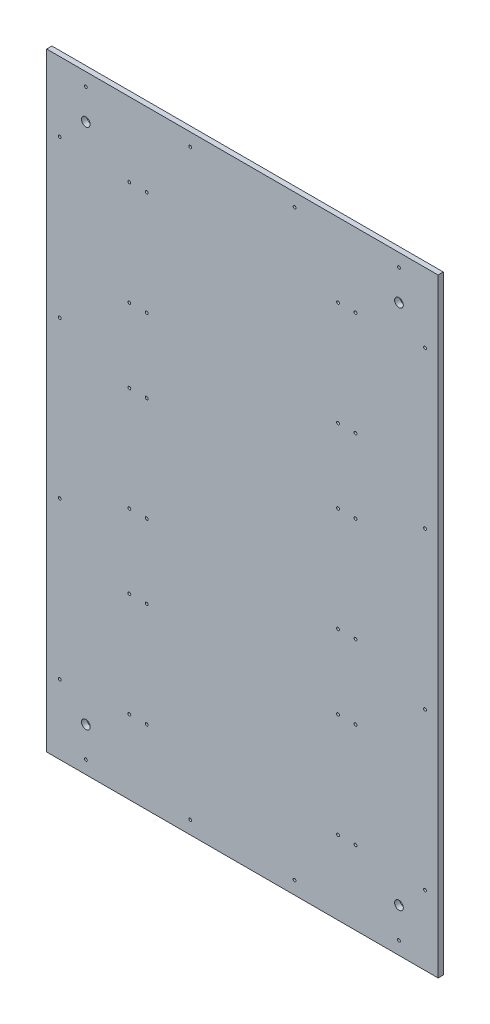
from build123d import *

# Parameters (mm, degrees)
SKETCH_1_W             = 450
SKETCH_1_H             = 700
EXTRUDE_1_DEPTH        = 6
HOLE_WIZARD_M4_1_D     = 3.3
HOLE_WIZARD_M4_1_DEPTH = 27.1
HOLE_WIZARD_M4_1_TIP   = 0.991420021
HOLE_WIZARD_M4_2_D     = 3.3
HOLE_WIZARD_M4_2_DEPTH = 27.1
HOLE_WIZARD_M4_2_TIP   = 0.991420021
SKETCH_7_R             = 5
CUT_EXTRUDE_1_DEPTH    = 10


with BuildPart() as part:
    # 草图1 → 凸台-拉伸1 (new body)
    with BuildSketch(Plane.XY):
        Rectangle(SKETCH_1_W, SKETCH_1_H)
    extrude(amount=EXTRUDE_1_DEPTH)

    # M4 螺纹孔1
    with Locations(Plane.XY.offset(6)):
        with Locations((130, -265), (110, -265), (110, -145), (130, -145), (110, -60), (130, -60), (130, 60), (110, 60), (-130, -265), (-110, -265), (-130, -145), (-110, -145), (-130, -60), (-110, -60), (-130, 60), (-110, 60), (-130, 145), (-110, 145), (-130, 265), (-110, 265), (110, 145), (130, 145), (110, 265), (130, 265)):
            Hole(HOLE_WIZARD_M4_1_D / 2, depth=HOLE_WIZARD_M4_1_DEPTH)
            with Locations((0, 0, -(HOLE_WIZARD_M4_1_DEPTH + HOLE_WIZARD_M4_1_TIP / 2))):  # 118° drill point
                Cone(0, HOLE_WIZARD_M4_1_D / 2, HOLE_WIZARD_M4_1_TIP, mode=Mode.SUBTRACT)

    # M4 螺纹孔2
    with Locations(Plane.XY.offset(6)):
        with Locations((-180, 335), (-60, 335), (60, 335), (180, 335), (-180, -335), (-60, -335), (60, -335), (180, -335), (210, -270), (210, -90), (210, 90), (210, 270), (-210, 270), (-210, 90), (-210, -90), (-210, -270)):
            Hole(HOLE_WIZARD_M4_2_D / 2, depth=HOLE_WIZARD_M4_2_DEPTH)
            with Locations((0, 0, -(HOLE_WIZARD_M4_2_DEPTH + HOLE_WIZARD_M4_2_TIP / 2))):  # 118° drill point
                Cone(0, HOLE_WIZARD_M4_2_D / 2, HOLE_WIZARD_M4_2_TIP, mode=Mode.SUBTRACT)

    # 草图7 → 切除-拉伸1 (cut)
    with BuildSketch(Plane.XY.offset(6)):
        with Locations((180, -300)):
            Circle(SKETCH_7_R)
        with Locations((-180, -300)):
            Circle(SKETCH_7_R)
        with Locations((-180, 300)):
            Circle(SKETCH_7_R)
        with Locations((180, 300)):
            Circle(SKETCH_7_R)
    extrude(amount=-CUT_EXTRUDE_1_DEPTH, mode=Mode.SUBTRACT)


solid = part.part
